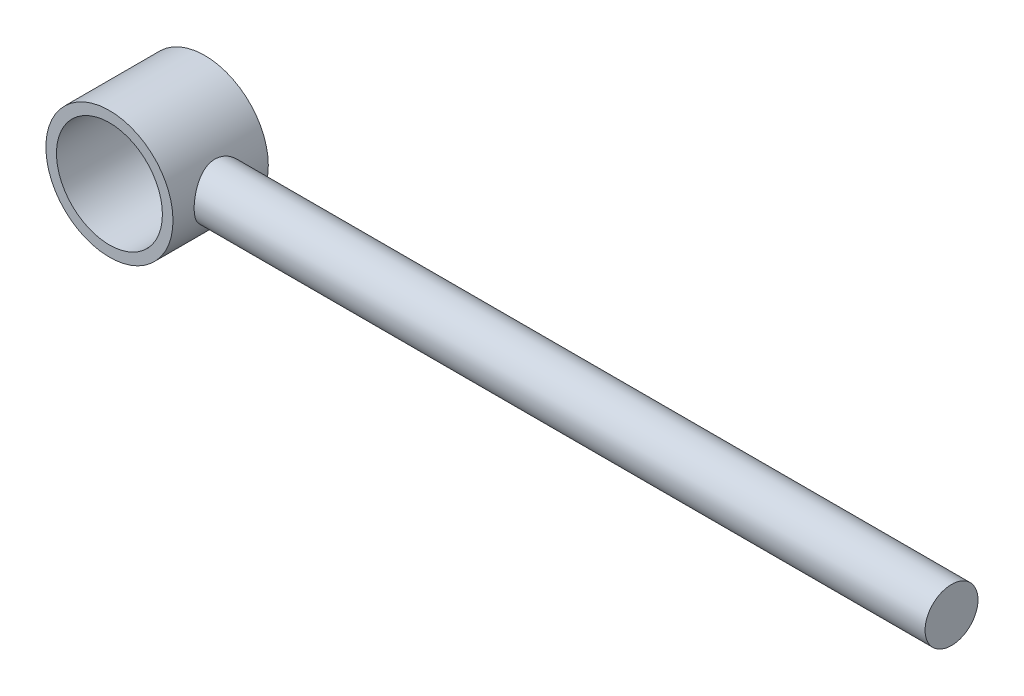
SolidWorks part; units mm, degrees
ref_plane "Front Plane" through (0, 0, 0) normal (0, 0, 1) x (1, 0, 0)
ref_plane "Top Plane" through (0, 0, 0) normal (0, 1, 0) x (1, 0, 0)
ref_plane "Right Plane" through (0, 0, 0) normal (1, 0, 0) x (0, 0, -1)
other "Configuration Table"
sketch "Sketch1" plane through (0, 0, 0) normal (0, 0, 1) x (1, 0, 0)
  circle A0 centre (0, 0) radius 10
  circle A1 centre (0, 0) radius 12
  dimension "D1" = 20
  dimension "D2" = 24
extrude "Boss-Extrude1" add sketch "Sketch1" along normal mid plane 18
ref_plane "Plane1" through (150, 0, 0) normal (1, 0, 0) x (0, 0, -1)
sketch "Sketch2" plane through (150, 0, 0) normal (1, 0, 0) x (0, 0, -1)
  circle A0 centre (0, 0) radius 5
  dimension "D1" = 10
extrude "Boss-Extrude2" add sketch "Sketch2" against normal up to next
